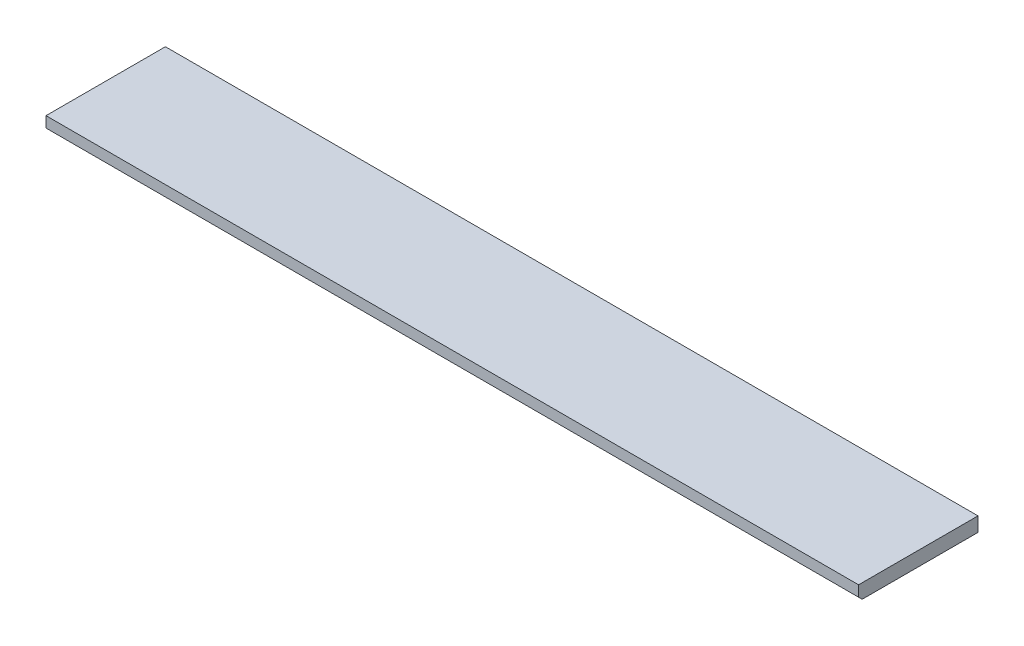
SolidWorks part; units mm, degrees
ref_plane "前视基准面" through (0, 0, 0) normal (0, 0, 1) x (1, 0, 0)
ref_plane "上视基准面" through (0, 0, 0) normal (0, 1, 0) x (1, 0, 0)
ref_plane "右视基准面" through (0, 0, 0) normal (1, 0, 0) x (0, 0, -1)
sketch "草图1" plane through (0, 0, 0) normal (0, 1, 0) x (1, 0, 0)
  line L1 (-1133, -166.5) -> (1133, -166.5)
  line L2 (-1133, -166.5) -> (-1133, 166.5)
  line L3 (-1133, 166.5) -> (1133, 166.5)
  line L4 (1133, -166.5) -> (1133, 166.5)
  line L5 (-1133, -166.5) -> (1133, 166.5) construction
  line L6 (-1133, 166.5) -> (1133, -166.5) construction
  point P0 (0, 0)
  dimension "D1" = 333
  dimension "D2" = 2266
extrude "凸台-拉伸1" add sketch "草图1" along normal blind 40
chamfer "倒角1" distance 10 angle 45 1 edges at (0, 0, 166.5)
